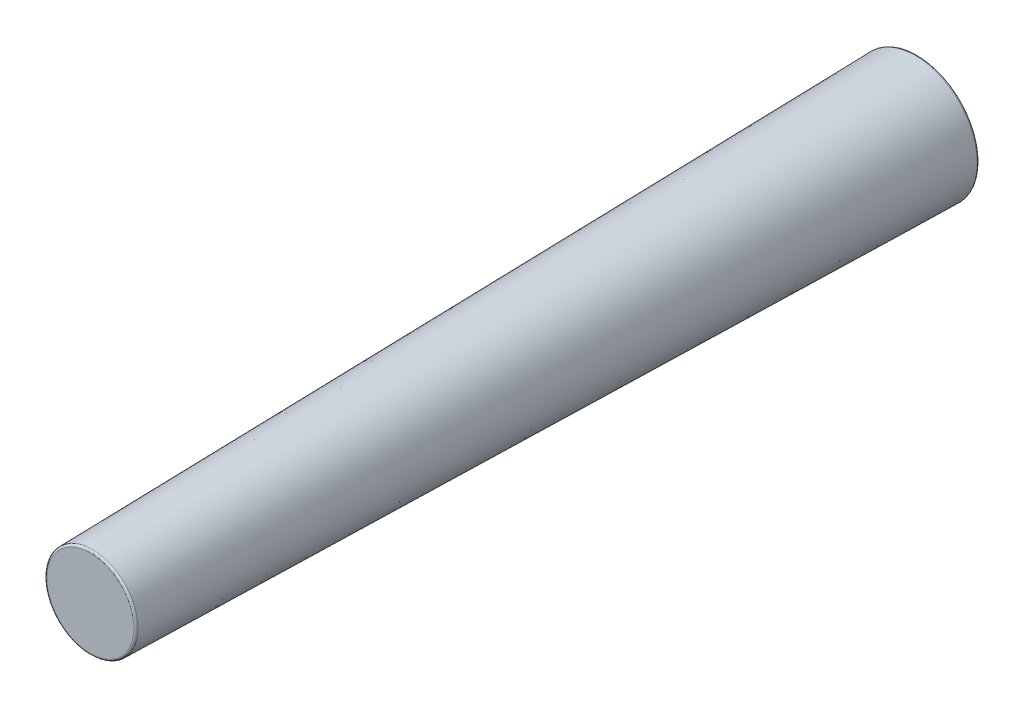
SolidWorks part; units mm, degrees
ref_plane "前视基准面" through (0, 0, 0) normal (0, 0, 1) x (1, 0, 0)
ref_plane "上视基准面" through (0, 0, 0) normal (0, 1, 0) x (1, 0, 0)
ref_plane "右视基准面" through (0, 0, 0) normal (1, 0, 0) x (0, 0, -1)
sketch "草图1" plane through (0, 0, 0) normal (0, 0, 1) x (1, 0, 0)
  circle A0 centre (0, 0) radius 3
  dimension "D1" = 6
extrude "凸台-拉伸1" add sketch "草图1" along normal blind 40 draft 1.14
fillet "圆角1" radius 0.1 2 edges at (3, 0, 0) (2.204, 0, 40)
